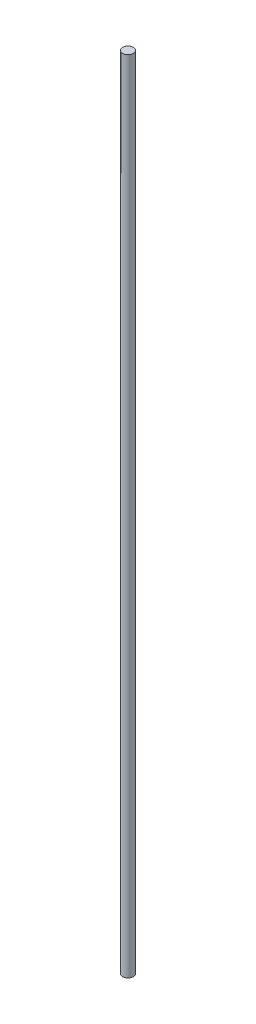
SolidWorks part; units mm, degrees
ref_plane "前视基准面" through (0, 0, 0) normal (0, 0, 1) x (1, 0, 0)
ref_plane "上视基准面" through (0, 0, 0) normal (0, 1, 0) x (1, 0, 0)
ref_plane "右视基准面" through (0, 0, 0) normal (1, 0, 0) x (0, 0, -1)
sketch "草图1" plane through (0, 0, 0) normal (0, 1, 0) x (1, 0, 0)
  circle A0 centre (0, 0) radius 2
  dimension "D1" = 4
extrude "凸台-拉伸1" add sketch "草图1" along normal blind 300
